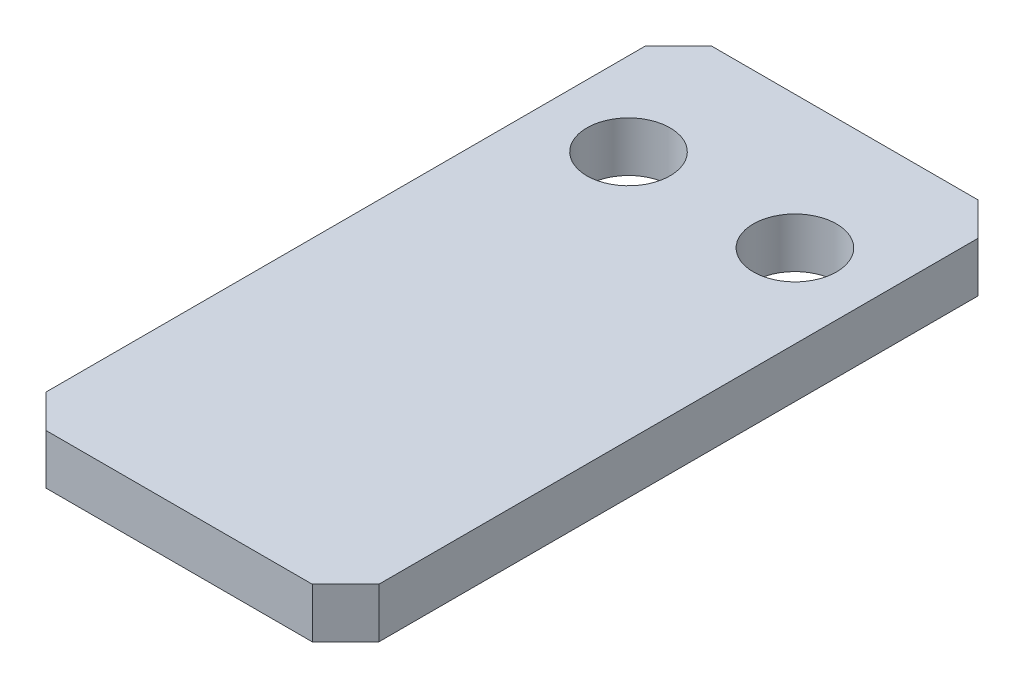
from build123d import *

# Parameters (mm, degrees)
SKETCH1_W                      = 10
SKETCH1_H                      = 20
BOSS_EXTRUDE1_DEPTH            = 1.5
CHAMFER1_SIZE                  = 1
F_2_5_2_5_DIAMETER_HOLE1_D     = 2.5
F_2_5_2_5_DIAMETER_HOLE1_DEPTH = 10
F_2_5_2_5_DIAMETER_HOLE1_TIP   = 0.751075774


with BuildPart() as part:
    # Sketch1 → Boss-Extrude1 (new body)
    with BuildSketch(Plane(origin=(0, 0, 0), x_dir=(1, 0, 0), z_dir=(0, 1, 0))):
        Rectangle(SKETCH1_W, SKETCH1_H)
    extrude(amount=BOSS_EXTRUDE1_DEPTH)

    # Chamfer1
    chamfer1_edges = [part.edges().sort_by_distance(p)[0] for p in [
        (5, 0.75, 10),
        (-5, 0.75, 10),
        (-5, 0.75, -10),
        (5, 0.75, -10),
    ]]
    chamfer(chamfer1_edges, length=CHAMFER1_SIZE)

    # Ø2.5 (2.5) Diameter Hole1
    with Locations(Plane(origin=(-2.5, 1.5, -6), x_dir=(0, 0, 1), z_dir=(0, 1, 0))):
        with Locations((0, 0), (0, 5)):
            Hole(F_2_5_2_5_DIAMETER_HOLE1_D / 2, depth=F_2_5_2_5_DIAMETER_HOLE1_DEPTH)
            with Locations((0, 0, -(F_2_5_2_5_DIAMETER_HOLE1_DEPTH + F_2_5_2_5_DIAMETER_HOLE1_TIP / 2))):  # 118° drill point
                Cone(0, F_2_5_2_5_DIAMETER_HOLE1_D / 2, F_2_5_2_5_DIAMETER_HOLE1_TIP, mode=Mode.SUBTRACT)


solid = part.part
